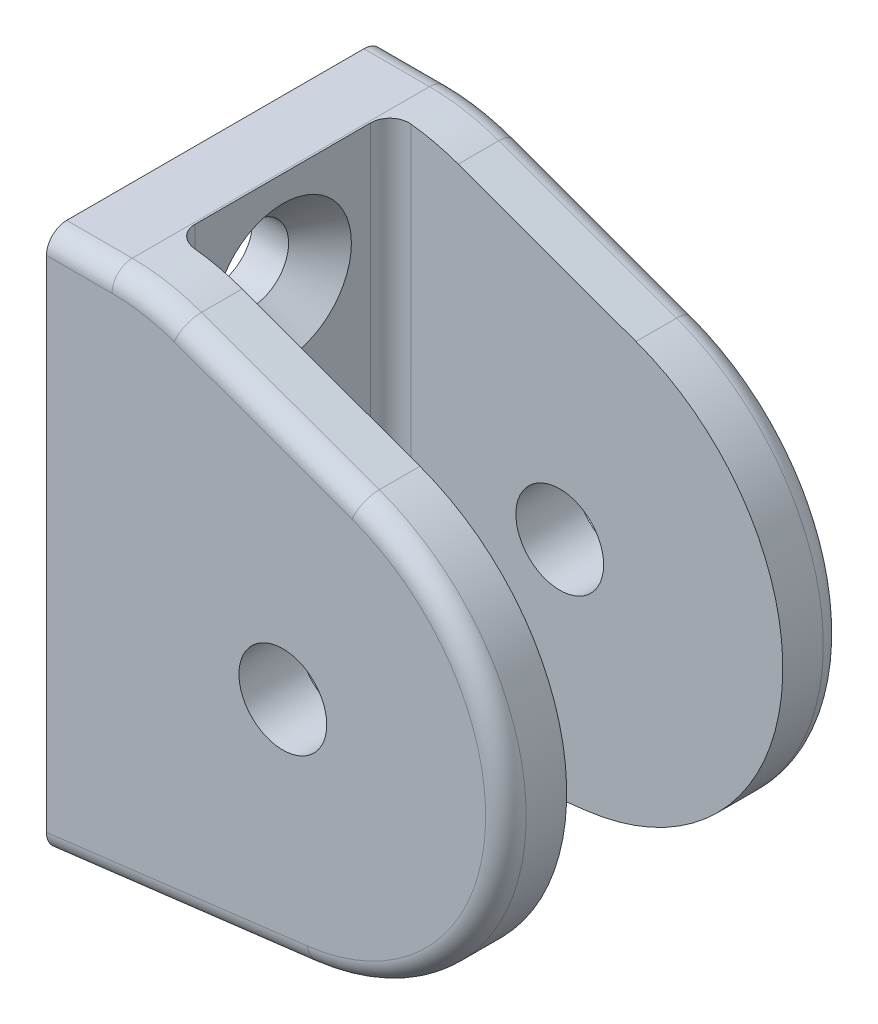
from build123d import *

# Parameters (mm, degrees)
EXTRUDE_1_DEPTH          = 25
SKETCH_3_W               = 68.112999437
SKETCH_3_H               = 98.020483962
CUT_EXTRUDE_1_DEPTH      = 16
SKETCH_4_R               = 6.5
CUT_EXTRUDE_2_DEPTH      = 117.308950023
FILLET_1_R               = 3
HOLE_WIZARD_1_AT_2_COUNT = 2
HOLE_WIZARD_1_AT_2_PITCH = 50.998600142
FILLET_2_R               = 3


with BuildPart() as part:
    # 草图2 → 凸台-拉伸1 (new, symmetric)
    with BuildSketch(Plane.XY):
        with BuildLine():
            Line((0, 0), (0, 80))
            Line((0, 80), (9.710190579, 80))
            ThreePointArc((9.710190579, 80), (14.919635909, 79.54423259), (19.970794879, 78.190778624))
            Line((19.970794879, 78.190778624), (46.296148462, 68.609133513))
            ThreePointArc((46.296148462, 68.609133513), (67.815421572, 33.834375668), (39.025067596, 4.791675789))
            Line((39.025067596, 4.791675789), (0, 0))
        make_face()
    extrude(amount=EXTRUDE_1_DEPTH, both=True)

    # 草图3 → 切除-拉伸1 (cut, symmetric)
    with BuildSketch(Plane.XY):
        with Locations((44.056499718, 41.123691615)):
            Rectangle(SKETCH_3_W, SKETCH_3_H)
    extrude(amount=CUT_EXTRUDE_1_DEPTH, both=True, mode=Mode.SUBTRACT)

    # 草图4 → 切除-拉伸2 (cut, through all)
    with BuildSketch(Plane.XY.offset(25)):
        with Locations((35, 37.573220687)):
            Circle(SKETCH_4_R)
    extrude(amount=-CUT_EXTRUDE_2_DEPTH, mode=Mode.SUBTRACT)

    # 圆角1
    fillet_1_edges = [part.edges().sort_by_distance(p)[0] for p in [
        (33.13347167, 73.399956068, 25),
        (14.919635909, 79.54423259, 25),
        (4.855095289, 80, 25),
        (19.512533798, 2.395837894, 25),
        (4.855095289, 80, -25),
        (14.919635909, 79.54423259, -25),
        (67.815421572, 33.834375668, 25),
        (33.13347167, 73.399956068, -25),
        (67.815421572, 33.834375668, -25),
        (19.512533798, 2.395837894, -25),
    ]]
    fillet(fillet_1_edges, radius=FILLET_1_R)

    # 草图6 → 打孔尺寸(%根据)内六角花形半沉头螺钉的类型1 (revolve, cut)
    with BuildSketch(Plane(origin=(10, 65.998600142, 0), x_dir=(0, 0, -1), z_dir=(0, 1, 0))):
        Polygon((0, 0), (0, 10), (5.5, 10), (5.5, 4.65), (10.15, 0), align=None)
    hole_wizard_1 = revolve(axis=Axis((16.35, 65.998600142, 0), (-1, 0, 0)), mode=Mode.SUBTRACT)

    # 打孔尺寸(%根据)内六角花形半沉头螺钉的类型1 at 2: 打孔尺寸(%根据)内六角花形半沉头螺钉的类型1 ×2
    with Locations(*[(0, -i * HOLE_WIZARD_1_AT_2_PITCH, 0) for i in range(1, HOLE_WIZARD_1_AT_2_COUNT)]):
        add(hole_wizard_1, mode=Mode.SUBTRACT)

    # 圆角2
    fillet_2_edges = [part.edges().sort_by_distance(p)[0] for p in [
        (10, 40.613222876, -16),
        (10, 40.613222876, 16),
    ]]
    fillet(fillet_2_edges, radius=FILLET_2_R)


solid = part.part
